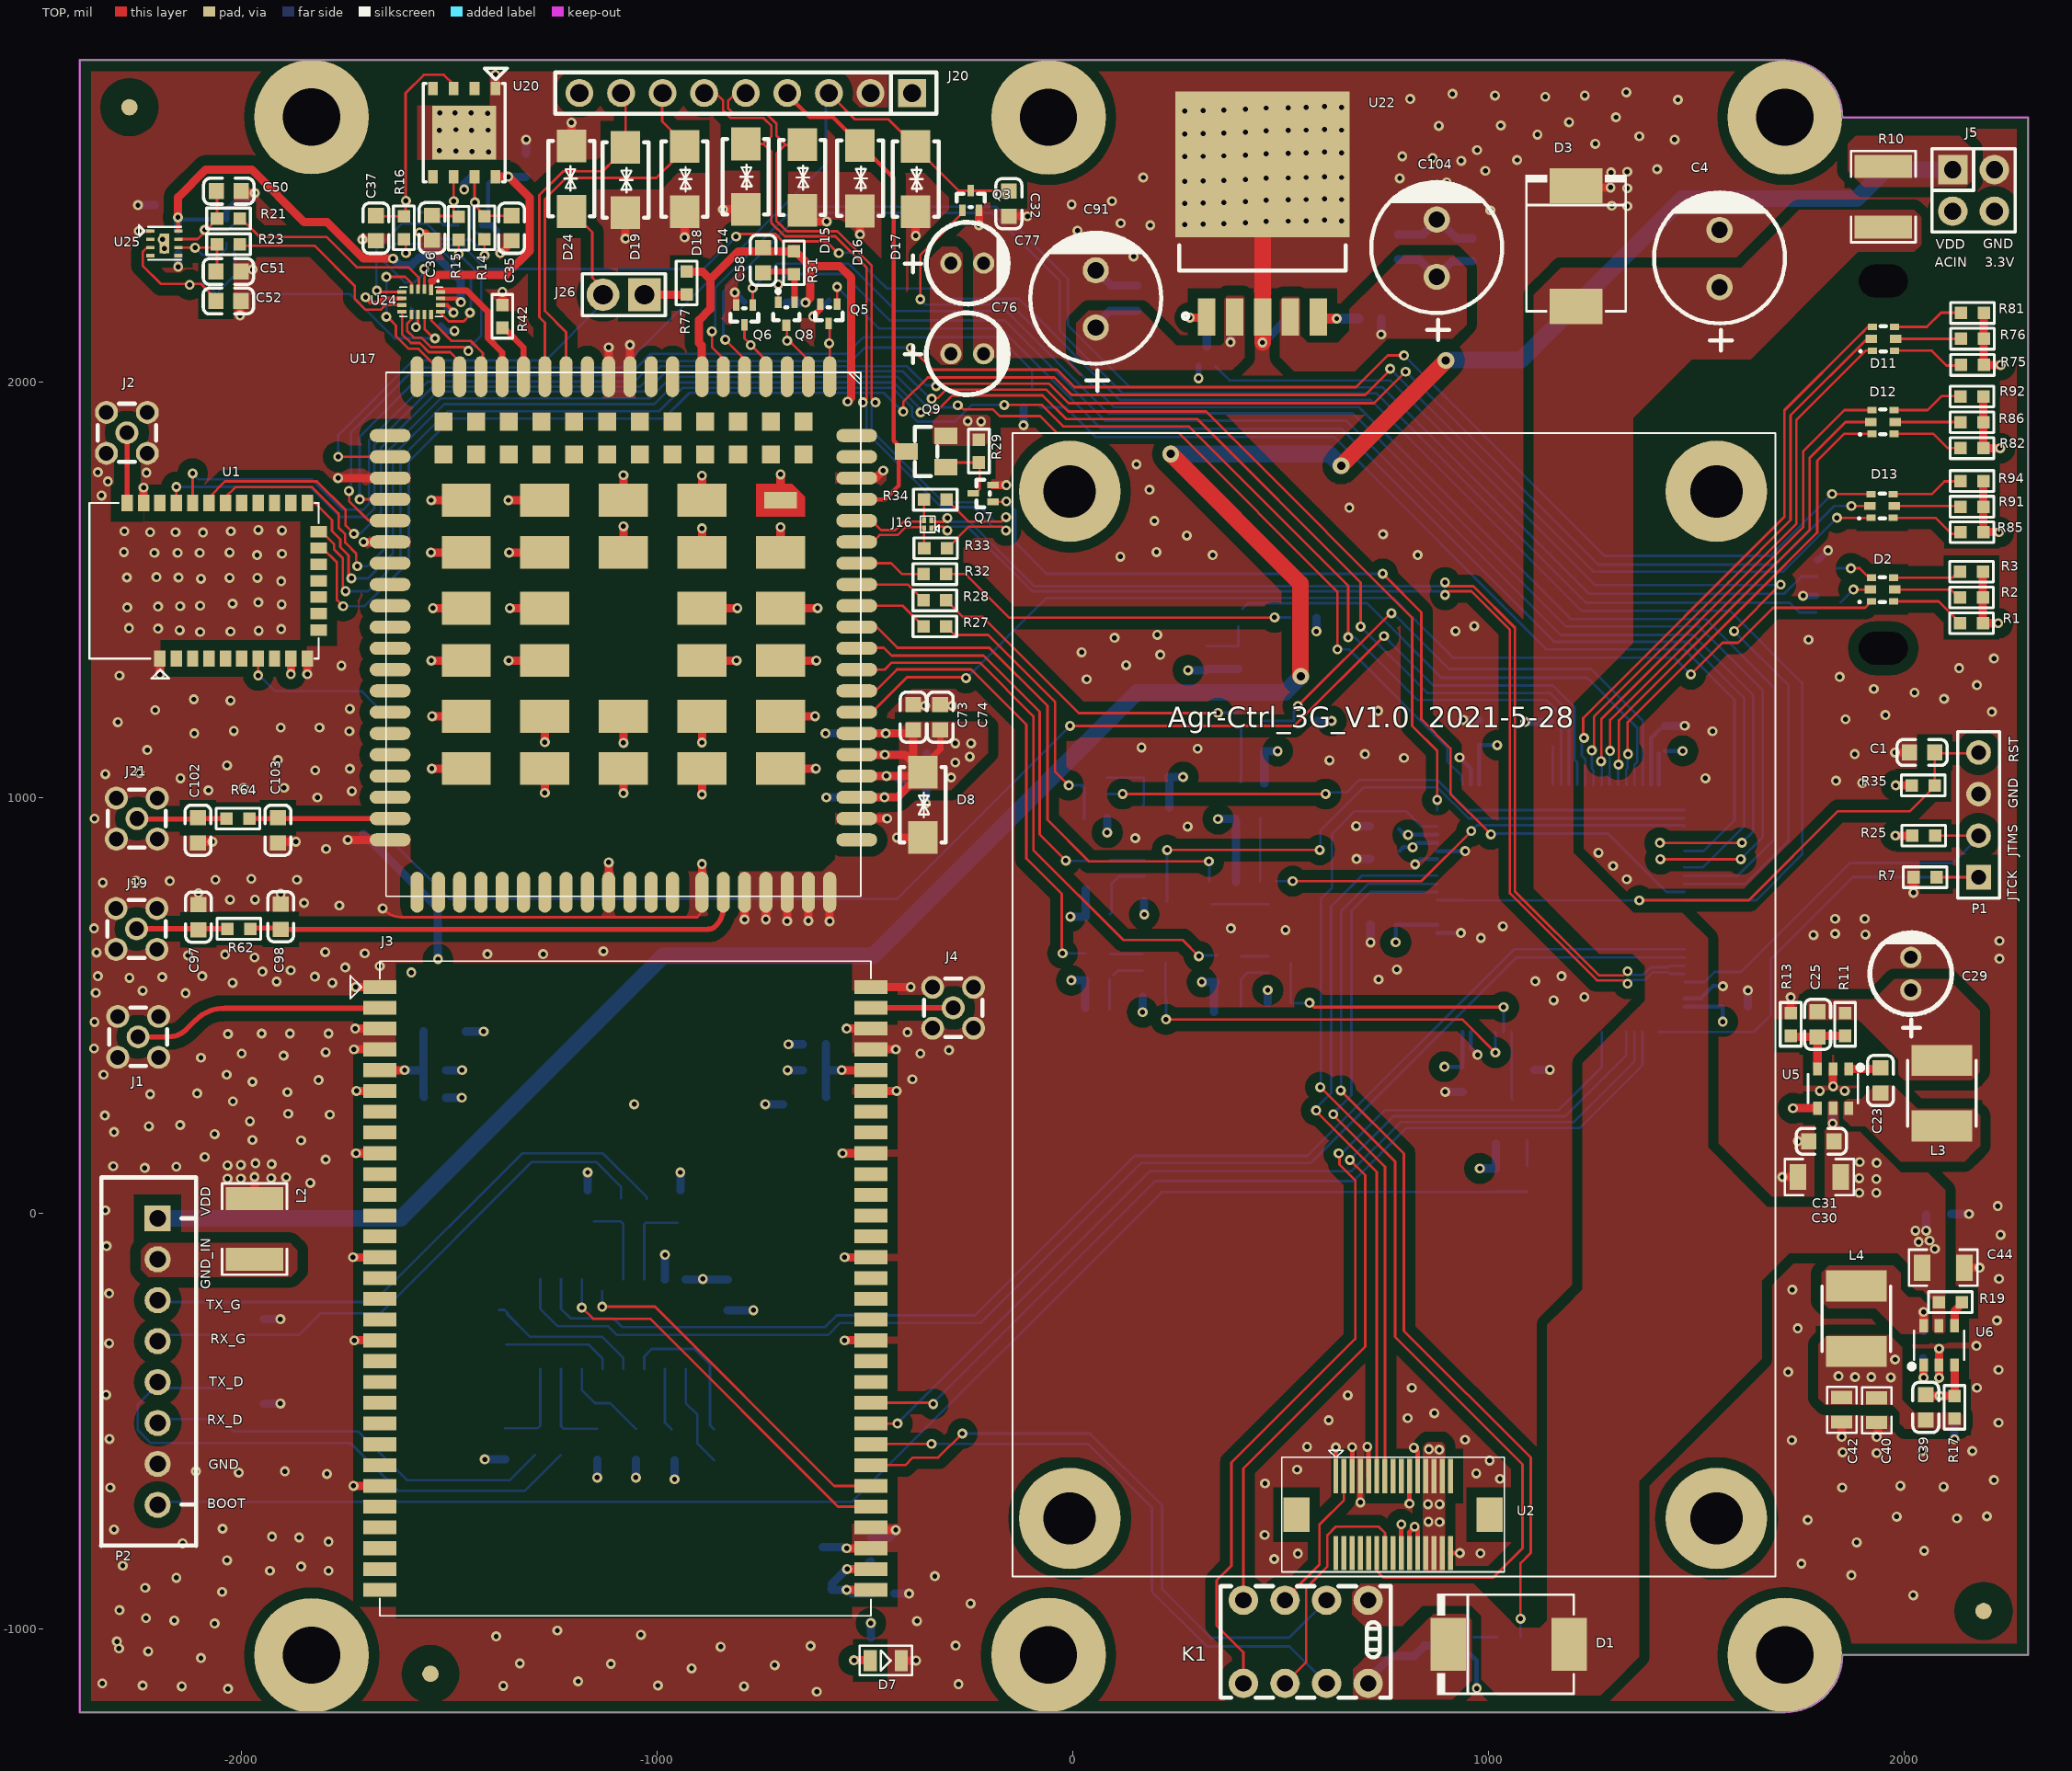
[diagram p0: TOP view]
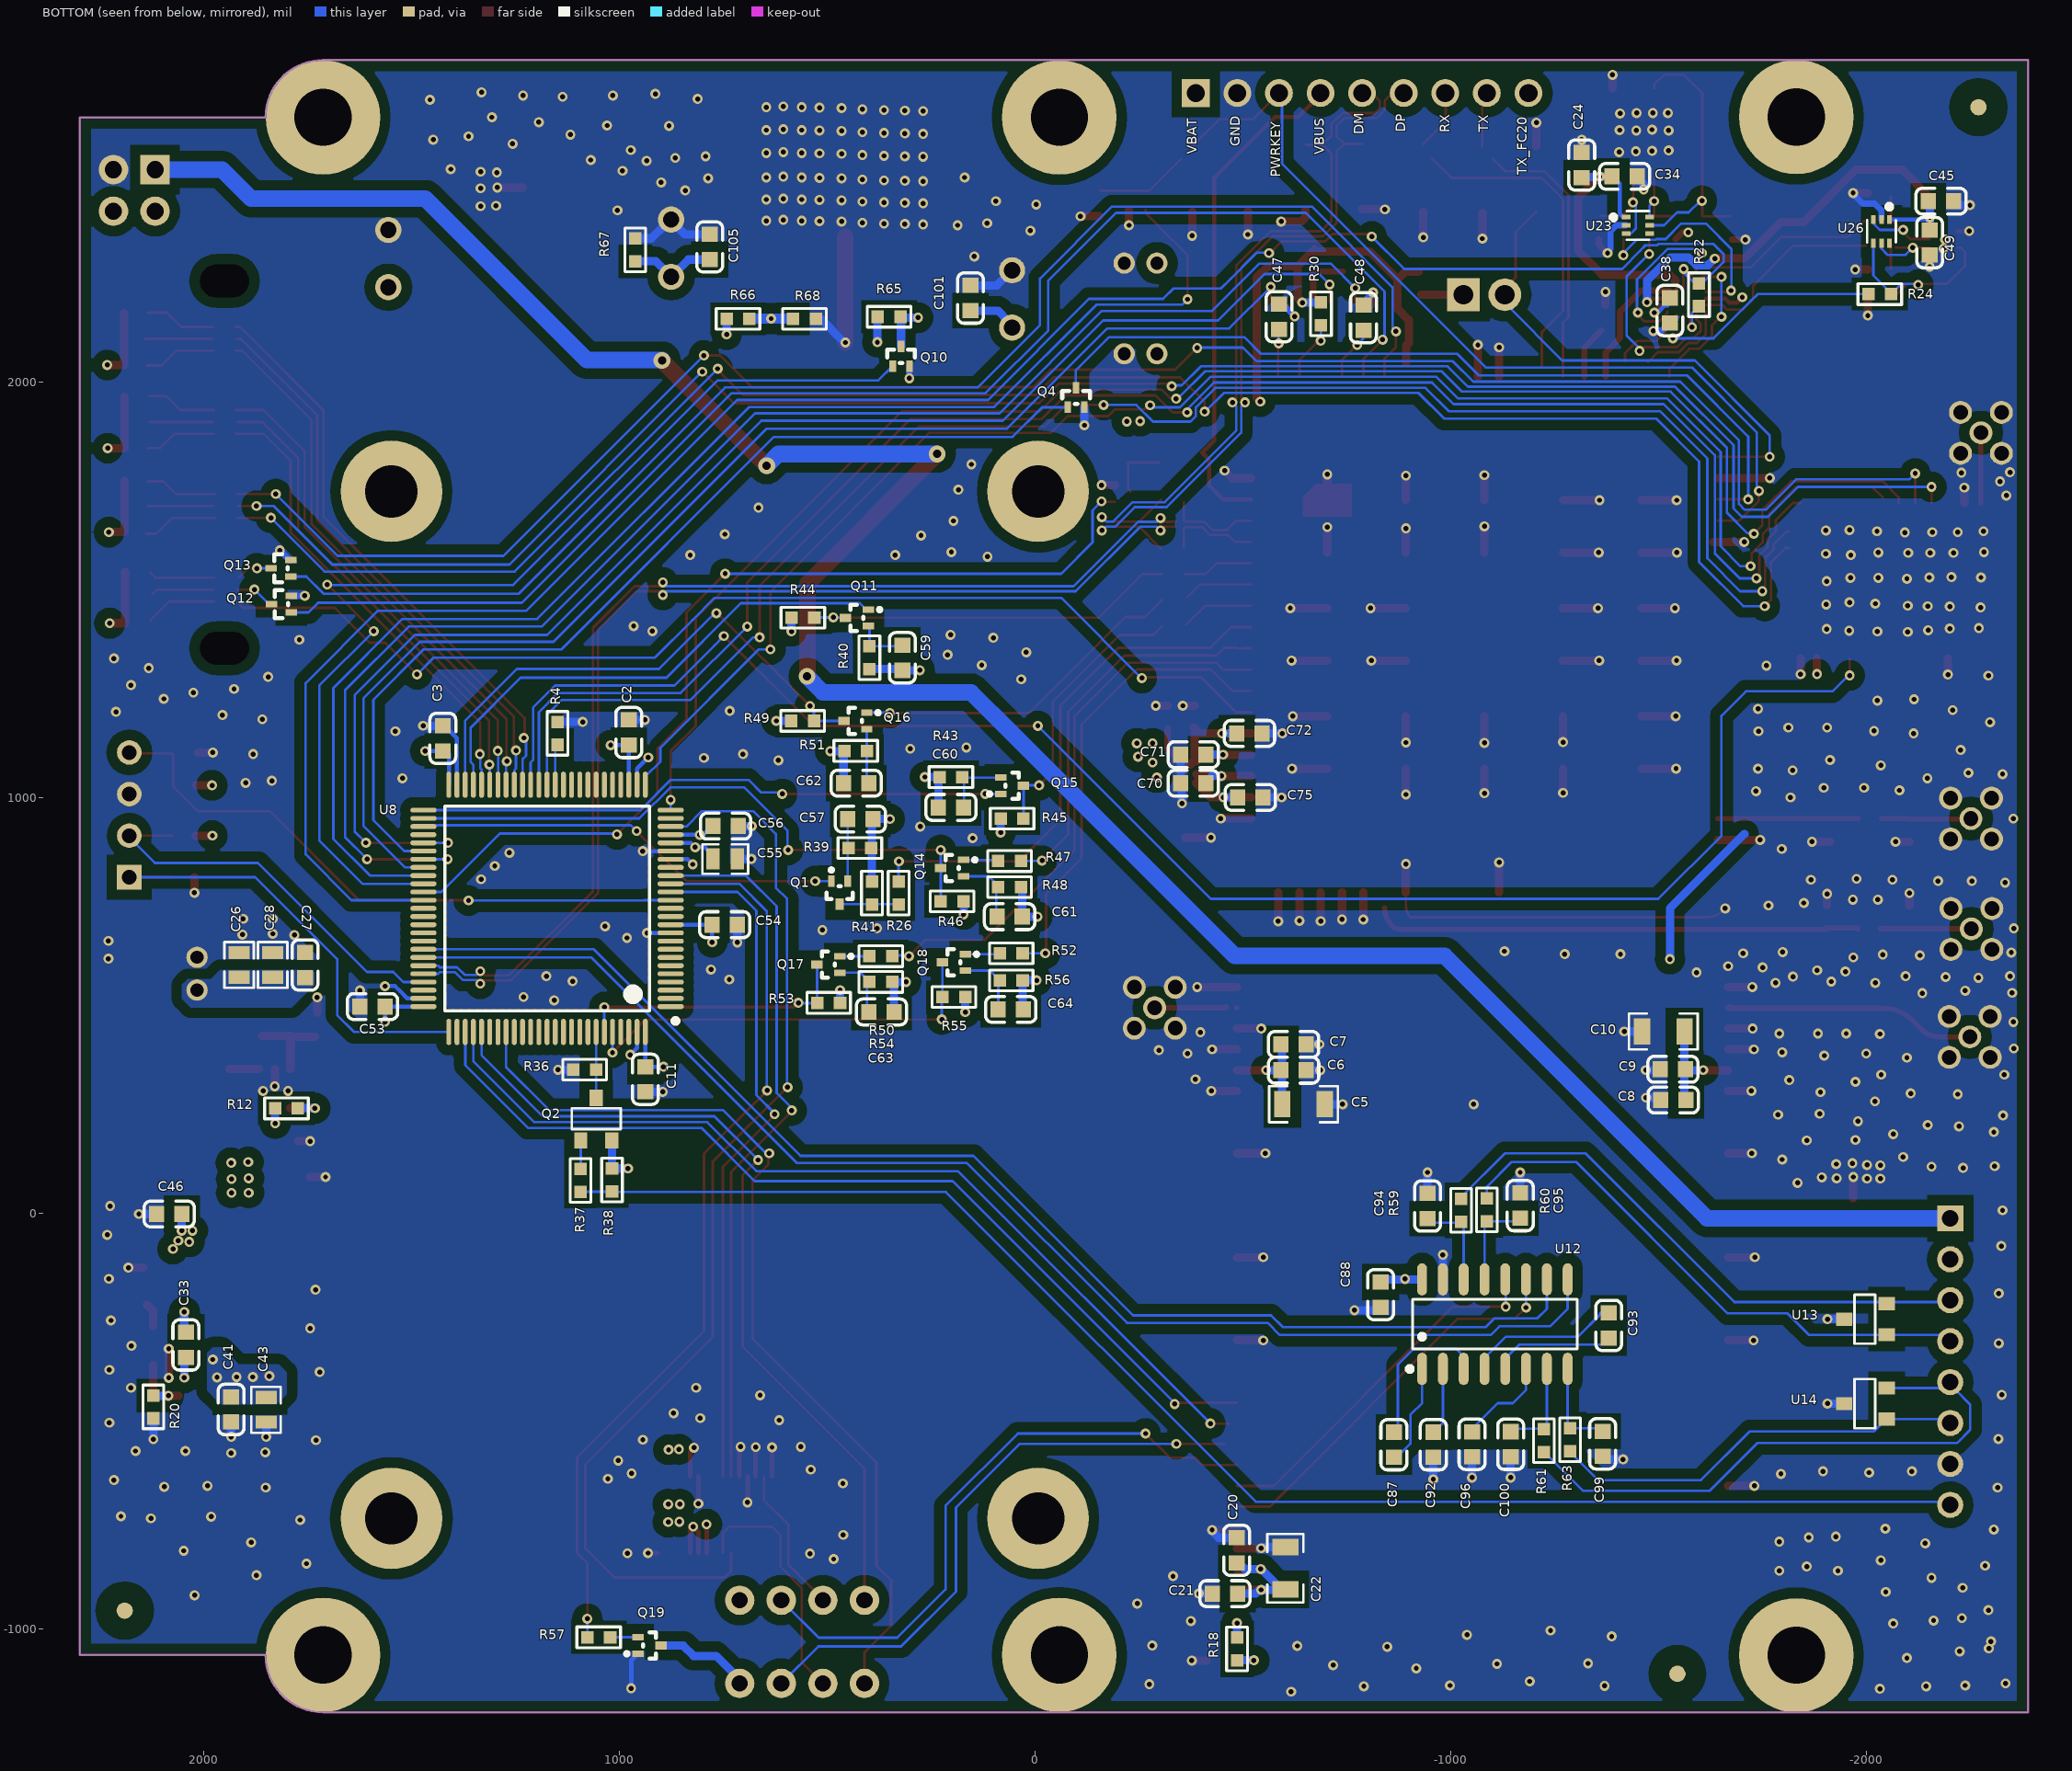
[diagram p1: BOTTOM view, seen from below]
# Altium PCB MISC84456.PcbDoc (part 1 of 5)
Units mil, origin at the board's own origin, x right, y up, seen from the top; angles counter-clockwise.
Board outline 4685.04 x 3973.82 mil, 4 copper layers (TOP, GND, POWER, BOTTOM), stack 38.4 mil thick; 219 components, 175 nets, 938 pads, 792 vias.

## Layer stack, top to bottom
TOP: signal copper 1.2
Dielectric: core 8, FR-4, Dk 4.5
GND: plane copper 1.4, net GND
Dielectric: prepreg 12.6, FR-4, Dk 4.8
POWER: plane copper 1.4, net (Multiple Nets)
Dielectric: core 12.6, FR-4, Dk 4.8
BOTTOM: signal copper 1.2

## Board outline
-2388.16,-1199.51 -2388.16,2774.31 1712.6,2774.31 cw(c1712.6,2636.52) 1850.39,2636.52 2296.88,2636.52 2296.88,-1061.71 1850.39,-1061.71 cw(c1712.6,-1061.71) 1712.6,-1199.51

## Design rules (kind name [scope] priority, off if disabled: settings)
Clearance Clearance_2 [haspad('free-MARK')] p1: gap=50
Clearance Clearance_1 [inpolygon] p2: gap=6
Clearance [All] p3: gap=6
DiffPairsRouting [All] p1: maxlimit=6 minlimit=6 mostfreqgap=6 maxuncoupledlength=500
HoleSize [All] p1: absolutevalues=TRUE maxlimit=500 minlimit=1 maxpercent=80.000 minpercent=20.000
HoleToHoleClearance [All] p1: gap=0 allowstackedmicrovias=TRUE
MinimumSolderMaskSliver [All] p1: minsoldermaskwidth=0
PlaneClearance [All] p1: clearance=10
PlaneConnect [All] p1: planeconnectstyle=Direct reliefexpansion=20 reliefentries=4 reliefconductorwidth=10 reliefairgap=10
PolygonConnect [All] p1: connectstyle=Direct reliefconductorwidth=10 reliefentries=4 polygonreliefangle="90 Angle"
RoutingVias [All] p1: holewidth=12 width=24 viastyle="Through Hole" minholewidth=12 minwidth=24 maxholewidth=12 maxwidth=24
SilkToSilkClearance [All] p1: silktosilkclearance=0
SilkscreenOverComponentPads [IsPad] p1: minsilkscreentomaskgap=0
SolderMaskExpansion [All] p1: expansion=4
Width [All] p1: maxlimit=40 minlimit=6 preferedwidth=6 minimp=151.900000 maximp=151.900000 favimp=151.900000
20 further rules are at their usual default settings.

## Classes and differential pairs
differential pair NewDifferentialPair2: +USB-DM2 -USB-DP2
differential pair NewDifferentialPair1: +USB_DM_TEST -USB_DP_TEST

## Components (designator, comment, footprint, x,y, rotation, side; value= is the part's Value field where it differs from the comment)
C1 "100nF/50V" C0603 2042,1109 r0 top
C2 "100nF/50V" C0603 977,1157 r90 bottom
C3 "100nF/50V" C0603 1424,1143 r90 bottom
C4 "470uF/25V" RB8*11.5 1555,2297 r90 top
C5 "10uF/25V±10%" C1206 -646,263 r0 bottom
C6 "100nF/50V" C0603 -622.12,344.76 r180 bottom
C7 "100pF" C0603 -622,407 r180 bottom
C8 "100pF" C0603 -1535,273 r180 bottom
C9 "100nF/50V" C0603 -1534,347 r180 bottom
C10 "10uF/25V±10%" C1206 -1511,438 r180 bottom
C11 "100nF/50V" C0603 937,323 r270 bottom
C20 "100pF" C0603 -485,-810 r270 bottom
C21 "100nF/50V" C0603 -457,-914 r180 bottom
C22 "10uF/25V±10%" C1206 -602,-853 r270 bottom
C23 "100nF/50V" C0603 1942,320 r90 top
C24 "100nF/50V" C0603 -1315,2522 r90 bottom
C25 "100pF" C0603 1791,455 r270 top
C26 "22uF/10V±20%" C0805 1914,598 r90 bottom
C27 "100nF/50V" C0603 1755,598 r90 bottom
C28 "22uF/10V±20%" C0805 1833,598 r90 bottom
C29 "100uF/10V" RB5*7 2015,577 r90 top
C30 "10uF/25V±10%" C1206 1795,88 r0 top
C31 "100nF/50V" C0603 1800,174 r0 top
C32 "10nF/50V" C0603 -154,2429 r270 top
C33 "100nF/50V" C0603 2042,-316 r270 bottom
C34 "33pF/50V" C0603 -1418,2495 r180 bottom
C35 "33pF/50V" C0603 -1350,2370 r270 top
C36 "33pF/50V" C0603 -1541,2371 r270 top
C37 "33pF/50V" C0603 -1676,2370 r270 top
C38 "100nF/50V" C0603 -1527,2172 r90 bottom
C39 "100pF" C0603 2051,-466 r90 top
C40 "22uF/10V±20%" C0805 1933,-473 r270 top
C41 "100nF/50V" C0603 1933,-471 r270 bottom
C42 "22uF/10V±20%" C0805 1849,-472 r270 top
C43 "22uF/10V±20%" C0805 1849,-472 r270 bottom
C44 "10uF/25V±10%" C1206 2093,-130 r180 top
C45 "100nF/50V" C0603 -2179,2435 r180 bottom
C46 "100nF/50V" C0603 2082,-1 r180 bottom
C47 "10nF/50V" C0603 -587,2157 r90 bottom
C48 "10nF/50V" C0603 -790,2155 r90 bottom
C49 "33pF/50V" C0603 -2151.68,2335.56 r270 bottom
C50 "33pF/50V" C0603 -2030,2459 r0 top
C51 "33pF/50V" C0603 -2031,2266 r0 top
C52 "33pF/50V" C0603 -2031,2195 r0 top
C53 "100nF/50V" C0603 1593,498 r0 bottom
C54 "100nF/50V" C0603 746,695 r180 bottom
C55 "10nF/50V" C0805 745,853 r0 bottom
C56 "100nF/50V" C0603 744,932 r180 bottom
C57 "1nF/50V" C0603 420,949 r0 bottom
C58 "1nF/50V" C0603 -745,2293 r90 top
C59 "1nF/50V" C0603 319,1337 r90 bottom
C60 "1nF/50V" C0603 202,977 r180 bottom
C61 "1nF/50V" C0603 61,714 r180 bottom
C62 "1nF/50V" C0603 430,1035 r0 bottom
C63 "1nF/50V" C0603 369,485 r180 bottom
C64 "1nF/50V" C0603 58,491 r180 bottom
C70 "100nF/50V" C0603 -381,1035 r0 bottom
C71 "33pF/50V" C0603 -381,1104 r0 bottom
C72 "12pF/50V" C0603 -516,1155 r180 bottom
C73 "100nF/50V" C0603 -384,1194 r90 top
C74 "33pF/50V" C0603 -319,1194 r90 top
C75 "12pF/50V" C0603 -518,1001 r180 bottom
C76 "100uF/10V" RB5*7 -254,2068 r0 top
C77 "100uF/10V" RB5*7 -254,2286 r0 top
C87 "100nF/50V" C0603 -863,-556 r270 bottom
C88 "100nF/50V" C0603 -831,-195 r270 bottom
C91 "470uF/25V" RB8*11.5 55,2200 r90 top
C92 "100nF/50V" C0603 -958,-556 r270 bottom
C93 "100nF/50V" C0603 -1380,-269 r90 bottom
C94 "12pF/50V" C0603 -944,18.1 r270 bottom
C95 "12pF/50V" C0603 -1167,19.1 r270 bottom
C96 "100nF/50V" C0603 -1051,-555 r270 bottom
C97 "NM" C0603 -2103,713 r270 top
C98 "NM" C0603 -1905,714 r270 top
C99 "12pF/50V" C0603 -1365,-553.9 r270 bottom
C100 "12pF/50V" C0603 -1144,-554.9 r270 bottom
C101 "100nF/50V" C0603 155,2202 r90 bottom
C102 "NM" C0603 -2104,922 r90 top
C103 "NM" C0603 -1912,922 r90 top
C104 "470uF/25V" RB8*11.5 875,2322 r90 top
C105 "100nF/50V" C0603 782,2325 r90 bottom
D1 "SMCJ18A" SMC 1048,-1036 r0 top
D2 "RGB" RGB 1947,1501 r180 top
D3 "SMCJ18A" SMC 1210,2327 r270 top
D7 "GREEN" LED0805 -450,-1075 r0 top
D8 "SMAJ6.8CA" SMA -361,983 r180 top
D11 "RGB" RGB 1949,2104 r180 top
D12 "RGB" RGB 1948,1904 r180 top
D13 "RGB" RGB 1946,1702 r180 top
D14 "SMAJ6.8CA" SMA -787,2494 r180 top
D15 "SMAJ6.8CA" SMA -651,2492 r180 top
D16 "SMAJ6.8CA" SMA -512,2490 r180 top
D17 "SMAJ6.8CA" SMA -378,2488 r180 top
D18 "SMAJ6.8CA" SMA -934,2488 r180 top
D19 "SMAJ6.8CA" SMA -1076,2486 r180 top
D24 "SMAJ6.8CA" SMA -1206,2489 r0 top
J1 "MMCX-KE RF connector" MMCX-KE -2248,425 r0 top
J2 "MMCX-KE RF connector" MMCX-KE -2275,1878 r270 top
J3 "UM482/K823" UM482/K823 -1076,-180 r0 top locked
J4 "MMCX-KE RF connector" MMCX-KE -288,495 r0 top
J5 "POWER" 2.54mm_2x2 2166,2461 r270 top
J16 "DLM0NSN900HY2D" SMD_0.85x0.65mm -349,1658 r180 top
J19 "MMCX-KE RF connector" MMCX-KE -2251.88,684.76 r0 top
J20 "2.54_9" 2.54-9P -786.75,2695.12 r180 top
J21 "MMCX-KE RF connector" MMCX-KE -2251,950 r0 top
J26 "2.54-2" 2.54mm-2P -1080,2210 r180 top
K1 "12V DPDT" "G6K-2P D12" 560,-1030 r180 top
L2 "120Ω ±25% @100MHz" 1812 -1968,-37 r90 top
L3 "2.2uH/2A" SMD,4x4x2.6mm 2089.57,289.53 r90 top
L4 "2.2uH/2A" SMD,4x4x2.6mm 1884,-253 r270 top
P1 "Header 4" HDR1X4 2178,809 r90 top
P2 "XH-8A" XH-8A -2201,-356 r270 top
Q1 "2SC4617TLQ" SOT-416F_L1.6-W0.8-P1.00-LS1.6-TR 470,772 r0 bottom
Q2 "8550" SOT-23 1055,227 r180 bottom
Q3 "DTC043ZEBTL" SOT-416_L1.6-W0.8-P1.00-LS1.6-BR -246,2432 r0 top
Q4 "DTC043ZEBTL" SOT-416_L1.6-W0.8-P1.00-LS1.6-BR -99,1958 r180 bottom
Q5 "DTC043ZEBTL" SOT-416_L1.6-W0.8-P1.00-LS1.6-BR -587.12,2169.25 r180 top
Q6 "DTC043ZEBTL" SOT-416_L1.6-W0.8-P1.00-LS1.6-BR -790.12,2166.25 r180 top
Q7 "DTC043ZEBTL" SOT-416_L1.6-W0.8-P1.00-LS1.6-BR -211,1732 r90 top
Q8 "2SC4617TLQ" SOT-416F_L1.6-W0.8-P1.00-LS1.6-TR -689,2164 r180 top
Q9 "SI2333CDS-T1-E3" SOT-23_L2.9-W1.3-P1.90-LS2.4-BR -353,1833 r90 top
Q10 "DTC043ZEBTL" SOT-416_L1.6-W0.8-P1.00-LS1.6-BR 322,2057 r180 bottom
Q11 "2SC4617TLQ" SOT-416F_L1.6-W0.8-P1.00-LS1.6-TR 428,1433 r90 bottom
Q12 "DTC043ZEBTL" SOT-416_L1.6-W0.8-P1.00-LS1.6-BR 1807,1466 r90 bottom
Q13 "DTC043ZEBTL" SOT-416_L1.6-W0.8-P1.00-LS1.6-BR 1808,1552 r90 bottom
Q14 "2SC4617TLQ" SOT-416F_L1.6-W0.8-P1.00-LS1.6-TR 199,831 r90 bottom
Q15 "2SC4617TLQ" SOT-416F_L1.6-W0.8-P1.00-LS1.6-TR 55,1029 r270 bottom
Q16 "2SC4617TLQ" SOT-416F_L1.6-W0.8-P1.00-LS1.6-TR 432,1185 r90 bottom
Q17 "2SC4617TLQ" SOT-416F_L1.6-W0.8-P1.00-LS1.6-TR 497,599 r90 bottom
Q18 "2SC4617TLQ" SOT-416F_L1.6-W0.8-P1.00-LS1.6-TR 195,604 r90 bottom
Q19 "2SC4617TLQ" SOT-416F_L1.6-W0.8-P1.00-LS1.6-TR 927,-1039 r270 bottom
R1 "1K5" R0603 2161,1420 r180 top
R2 "680R" R0603 2161,1482 r180 top
R3 "1K" R0603 2161,1544 r180 top
R4 "10K" R0603 1148,1155 r270 bottom
R7 "10K" R0603 2049,809 r180 top
R10 "12V/2A" R1812 1949,2446 r90 top
R11 "75K 1%" R0603 1857,455 r90 top
R12 "100K" R0603 1800,253 r0 bottom
R13 "10K" R0603 1726,455 r270 top
R14 "22R" R0603 -1415,2371 r90 top
R15 "22R" R0603 -1477,2370 r90 top
R16 "22R" R0603 -1609,2371 r90 top
R17 "100K" R0603 2120,-466 r270 top
R18 "1K" R0603 -486,-1047 r270 bottom
R19 "100K" R0603 2110,-213 r180 top
R20 "22.1K 1%" R0603 2120,-465 r90 bottom
R21 "22R" R0603 -2030.68,2393.56 r180 top
R22 "NM" R0603 -1597,2210 r270 bottom
R23 "22R" R0603 -2030.68,2331.56 r180 top
R24 "22R" R0603 -2031.68,2211.44 r180 bottom
R25 "10K" R0603 2046,909 r180 top
R26 "0R" R0603 328,771 r90 bottom
R27 "0R" R0603 -332,1412 r180 top
R28 "0R" R0603 -332,1475 r180 top
R29 "10K" R0603 -226,1834 r270 top
R30 "4.7K" R0603 -688,2164 r270 bottom
R31 "4.7K" R0603 -671,2287 r270 top
R32 "0R" R0603 -332,1538 r180 top
R33 "NM" R0603 -330,1600 r180 top
R34 "NM" R0603 -331,1717 r180 top
R35 "10K" R0603 2045,1030 r180 top
R36 "10K" R0603 1083,346 r180 bottom
R37 "10K" R0603 1093,80 r270 bottom
R38 "10K" R0603 1017,81 r90 bottom
R39 "4.7K" R0603 421,879 r180 bottom
R40 "4.7K" R0603 398,1337 r270 bottom
R41 "10K" R0603 392,771 r270 bottom
R42 "NM" R0603 -1372,2158 r270 top
R43 "4.7K" R0603 202,1050 r0 bottom
R44 "10K" R0603 558,1433 r180 bottom
R45 "10K" R0603 55,950 r180 bottom
R46 "10K" R0603 199,751 r180 bottom
R47 "0R" R0603 61,848 r180 bottom
R48 "4.7K" R0603 61,785 r0 bottom
R49 "10K" R0603 559,1185 r0 bottom
R50 "0R" R0603 371,619 r180 bottom
R51 "4.7K" R0603 431,1113 r180 bottom
R52 "0R" R0603 57,626 r180 bottom
R53 "10K" R0603 496,507 r180 bottom
R54 "4.7K" R0603 371,557 r0 bottom
R55 "10K" R0603 195,521 r180 bottom
R56 "4.7K" R0603 57,561 r0 bottom
R57 "4.7K" R0603 1049,-1019 r0 bottom
R59 "4.7Ω,±1%" R0603 -1025,8.1 r270 bottom
R60 "4.7Ω,±1%" R0603 -1087,9.1 r270 bottom
R61 "4.7Ω,±1%" R0603 -1224,-545.9 r90 bottom
R62 "0R" R0603 -2006,685 r180 top
R63 "4.7Ω,±1%" R0603 -1287,-543.9 r90 bottom
R64 "0R" R0603 -2008,950 r180 top
R65 "47K" R0603 351,2157 r0 bottom
R66 "100K" R0603 714,2152 r0 bottom
R67 "330R" R0603 961,2318 r270 bottom
R68 "47K" R0603 554,2152 r0 bottom
R75 "1K5" R0603 2163,2041 r180 top
R76 "680R" R0603 2163,2104 r180 top
R77 "4.7K" R0603 -929,2238 r270 top
R81 "1K" R0603 2163,2166 r180 top
R82 "1K5" R0603 2162,1841 r180 top
R85 "1K5" R0603 2162,1639 r180 top
R86 "680R" R0603 2162,1903 r180 top
R91 "680R" R0603 2162,1700 r180 top
R92 "1K" R0603 2162,1965 r180 top
R94 "1K" R0603 2162,1762 r180 top
U1 "HLK-B40" HLK-B40 -2044,1522 r90 top
U2 "24-5046-030-600-829" HX-DU1006D 770,-724 r180 top locked
U5 "SY8113B" TSOT-23-6 1828,300.65 r90 top
U6 "SY8113B" TSOT-23-6 2083,-317 r270 top
U8 "STM32F103VCT6" LQFP-100_14x14x05P 1173.35,734.12 r90 bottom
U12 "SP3232EEN" SOP16-6.6 -1106,-265.9 r90 bottom
U13 "PESD15VL2BT" SOT-23 -1997,-254 r90 bottom
U14 "PESD15VL2BT" SOT-23 -1997,-457 r90 bottom
U17 "EC20" EC20 -1081,1393 r270 top locked
U20 "SIM-A China Telecom eSIM" VQFN8 -1464,2600 r270 top
U22 "MIC29302WU" TO-263-5 456,2340 r0 top
U23 "ESDA6V8V6-6" SOT-563 -1450,2377 r180 bottom
U24 "FSA2567MPX" MLP-16 -1567,2193 r180 top
U25 "SIM-B China Mobile eSIM" DFN2*2-8 -2184.68,2333.56 r0 top
U26 "ESDA6V8V6-6" SOT-563 -2035.68,2362.56 r270 bottom

## Footprints (in the part's own frame and the unit in brackets; to place one, negate y for a bottom-side part, rotate by r counter-clockwise, add the part's x,y. Pads: shape width x height; smd on the part's side, far side on the other; paste and mask are expansions set on the pad)
2.54-9P [mm]
  rect 1.7x1.7 hole 1.1: 1(-10.16,0)
  round 1.7 hole 1.1: 2(-7.62,0) 3(-5.08,0) 4(-2.54,0) 5(0,0) 6(2.54,0) 7(5.08,0) 8(7.62,0) 9(10.16,0)
  silkscreen extent -11.64,-1.27 11.64,1.27
2.54mm-2P [mm]
  rect 2x2 hole 1.2: 1(-1.27,0)
  round 2 hole 1.2: 2(1.27,0)
  silkscreen extent -2.54,-1.27 2.54,1.27
2.54mm_2x2 [mm]
  rect 1.8x1.8 hole 1.05: 1(-1.27,-1.27)
  round 1.8 hole 1.05: 2(-1.27,1.27) 3(1.27,-1.27) 4(1.27,1.27)
  silkscreen extent -2.54,-2.54 2.54,2.54
1812 [mil]
  rect 55.38x137.76 smd: 1(-72.97,0) 2(72.97,0)
  silkscreen extent -110,-78 110,78
C0603 [mm]
  rect 0.93x0.98 smd: 1(-0.77,0) 2(0.77,0)
  silkscreen extent -1.53,-0.79 1.54,0.79, body extent -0.8,-0.4 0.8,0.4, height 0.3
C0805 [mm] "C0805"
  rect 0.8x1.3 smd: 1(-0.75,0) 2(0.75,0)
  silkscreen extent -1.4,-0.9 1.4,0.9
C1206 [mm] "C1206"
  rect 1x1.6 smd: 1(-1.299,0) 2(1.3,0)
  silkscreen extent -2.1,-1.1 2.1,1.1
DFN2*2-8 [mm]
  rect 0.5x0.2 smd: 1(-0.85,0.75) 2(-0.85,0.25) 3(-0.85,-0.25) 4(-0.85,-0.75) 5(0.85,-0.75) 6(0.85,-0.25) 7(0.85,0.25) 8(0.85,0.75)
  rect 0.6x1.2 smd: 9(0,0)
  silkscreen extent -1.56,-1 1,1.12
EC20 [mm]
  oval 2.5x0.8 smd mask+0.05: 1(-15.75,12.6) 2(-15.75,11.3) 3(-15.75,10) 4(-15.75,8.7) 5(-15.75,7.4) 6(-15.75,6.1) 7(-15.75,4.8) 8(-15.75,0.4) 9(-15.75,-0.9) 10(-15.75,-2.2) 11(-15.75,-3.5) 12(-15.75,-4.8) 13(-15.75,-6.1) 14(-15.75,-7.4) 15(-15.75,-8.7) 16(-15.75,-10) 17(-15.75,-11.3) 18(-15.75,-12.6) 37(15.75,-12.6) 38(15.75,-11.3) 39(15.75,-10) 40(15.75,-8.7) 41(15.75,-7.4) 42(15.75,-6.1) 43(15.75,-4.8) 44(15.75,-3.5) 45(15.75,-2.2) 46(15.75,-0.9) 47(15.75,0.4) 48(15.75,4.8) 49(15.75,6.1) 50(15.75,7.4) 51(15.75,8.7) 52(15.75,10) 53(15.75,11.3) 54(15.75,12.6) 141(-15.75,3) 142(-15.75,1.7) 143(15.75,1.7) 144(15.75,3)
  oval 0.8x2.5 smd mask+0.05: 19(-9.55,-14.25) 20(-8.25,-14.25) 21(-6.95,-14.25) 22(-5.65,-14.25) 23(-4.35,-14.25) 24(-3.05,-14.25) 25(-1.75,-14.25) 26(-0.45,-14.25) 27(0.85,-14.25) 28(2.15,-14.25) 29(3.45,-14.25) 30(4.75,-14.25) 31(6.05,-14.25) 32(7.35,-14.25) 33(8.65,-14.25) 34(9.95,-14.25) 35(11.25,-14.25) 36(12.55,-14.25) 55(12.55,14.25) 56(11.25,14.25) 57(9.95,14.25) 58(8.65,14.25) 59(7.35,14.25) 60(6.05,14.25) 61(4.75,14.25) 62(3.45,14.25) 63(2.15,14.25) 64(0.85,14.25) 65(-0.45,14.25) 66(-1.75,14.25) 67(-3.05,14.25) 68(-4.35,14.25) 69(-5.65,14.25) 70(-6.95,14.25) 71(-8.25,14.25) 72(-9.55,14.25) 113(-10.85,14.25) 114(-12.15,14.25) 115(-10.85,-14.25) 116(-12.15,-14.25)
  rect 2x3 smd mask+0.05: 85(8.2,9.6) 86(8.2,4.8) 87(8.2,0) 88(8.2,-4.8) 89(8.2,-9.6) 90(5,9.6) 91(5,4.8) 92(5,0) 93(5,-4.8) 94(5,-9.6) 95(1.6,9.6) 96(1.6,4.8) 97(1.6,-4.8) 98(1.6,-9.6) 99(-1.6,9.6) 100(-1.6,4.8) 101(-1.6,-4.8) 102(-1.6,-9.6) 103(-5,9.6) 104(-5,4.8) 105(-5,0) 106(-5,-4.8) 107(-5,-9.6) 109(-8.2,4.8) 110(-8.2,0) 111(-8.2,-4.8) 112(-8.2,-9.6)
  rect 1x2 smd: 108(-8.2,9.6)
  rect 1.1x1.1 smd mask+0.05: 117(-11,11) 118(-11,9) 119(-11,7) 120(-11,5) 121(-11,3) 122(-11,1) 123(-11,-1) 124(-11,-3) 125(-11,-5) 126(-11,-7) 127(-11,-9) 128(-11,-11) 129(-13,11) 130(-13,9) 131(-13,7) 132(-13,5) 133(-13,3) 134(-13,1) 135(-13,-1) 136(-13,-3) 137(-13,-5) 138(-13,-7) 139(-13,-9) 140(-13,-11)
  TOP region: -9.2,10.3 -8.4,11.1 -7.2,11.1 -7.2,8.1 -9.2,8.1 -9.2,10.3
  TOP pour cut-out: 3.5,2.8 -3.5,2.8 -3.5,-2.8 3.5,-2.8 3.5,2.8
  silkscreen extent -16,-14.5 16,14.5